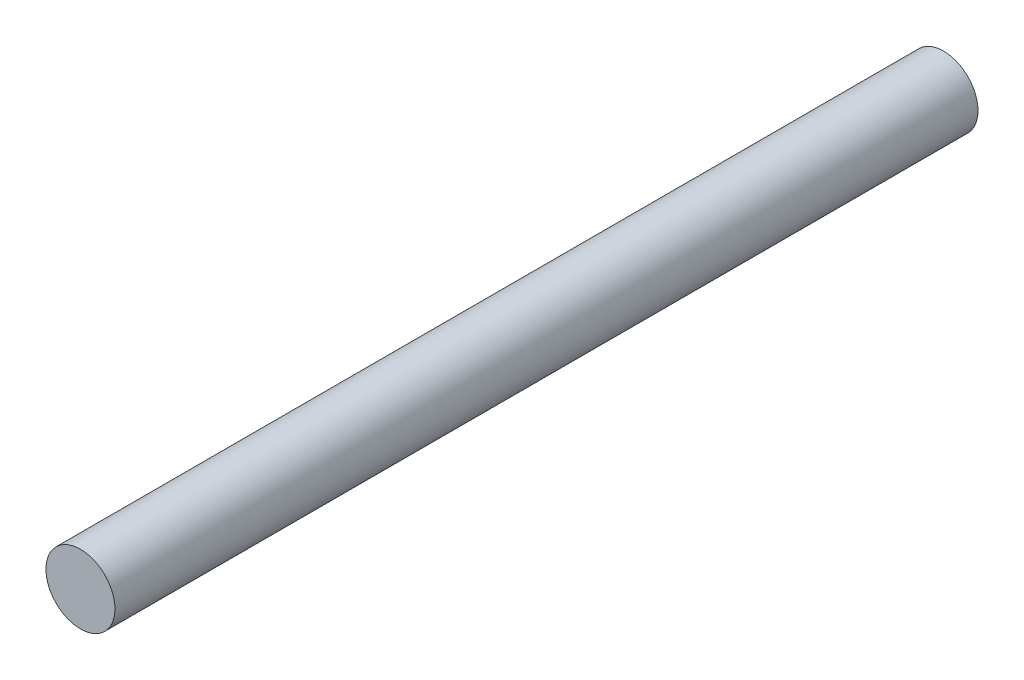
from build123d import *

# Parameters (mm, degrees)
SKETCH1_R           = 8
BOSS_EXTRUDE1_DEPTH = 200


with BuildPart() as part:
    # Sketch1 → Boss-Extrude1 (new body)
    with BuildSketch(Plane.XY):
        Circle(SKETCH1_R)
    extrude(amount=BOSS_EXTRUDE1_DEPTH)


solid = part.part
